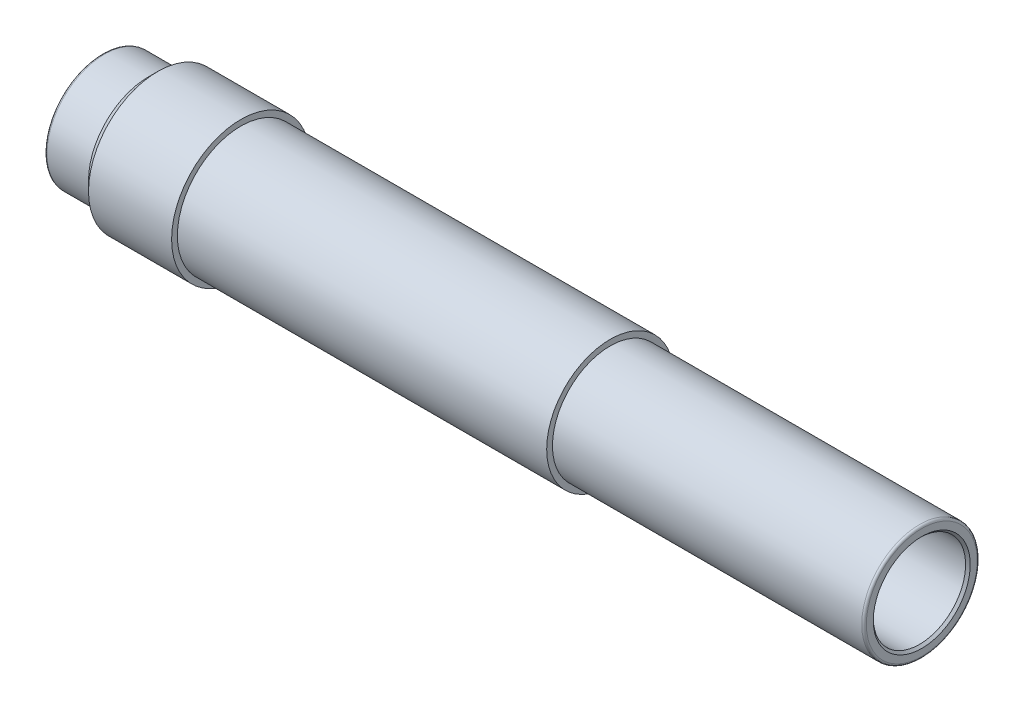
SolidWorks part; units mm, degrees
material "20钢"
ref_plane "Front Plane" through (0, 0, 0) normal (0, 0, 1) x (1, 0, 0)
ref_plane "Top Plane" through (0, 0, 0) normal (0, 1, 0) x (1, 0, 0)
ref_plane "Right Plane" through (0, 0, 0) normal (1, 0, 0) x (0, 0, -1)
other "Configuration Table"
sketch "Sketch 1" plane through (0, 0, 0) normal (0, 1, 0) x (1, 0, 0)
  line L0 (20, 26) -> (24, 30)
  line L1 (0, 0) -> (20, 0)
  line L2 (0, 0) -> (0, 25)
  line L4 (20, 0) -> (20, 25)
  line L5 (20, 0) -> (60, 0)
  line L6 (20, 0) -> (20, 26)
  line L7 (24, 30) -> (60, 30)
  line L8 (60, 0) -> (60, 30)
  line L9 (60, 0) -> (220, 0)
  line L10 (60, 0) -> (60, 27.5)
  line L11 (60, 27.5) -> (220, 27.5)
  line L12 (220, 0) -> (220, 27.5)
  line L13 (220, 0) -> (355, 0)
  line L14 (220, 0) -> (220, 25)
  line L15 (220, 25) -> (355, 25)
  line L16 (355, 0) -> (355, 25)
  line L17 (0, 0) -> (355, 0)
  line L18 (0, 0) -> (0, 20)
  line L19 (0, 20) -> (355, 20)
  line L20 (355, 0) -> (355, 20)
  line L21 (0, 25) -> (20, 25)
  point P6 (20, 30)
  dimension "D1" = 25
  dimension "D2" = 30
  dimension "D3" = 27.5
  dimension "D4" = 25
  dimension "D5" = 40
  dimension "D6" = 160
  dimension "D7" = 135
  dimension "D8" = 355
  dimension "D9" = 20
revolve "Revolve3" add sketch "Sketch 1" angle 360 about L5
fillet "Fillet1" radius 1 2 edges at (355, 0, 25) (0, 0, 25)
chamfer "Chamfer1" distance 1 angle 45 1 edges at (355, 0, 20)
